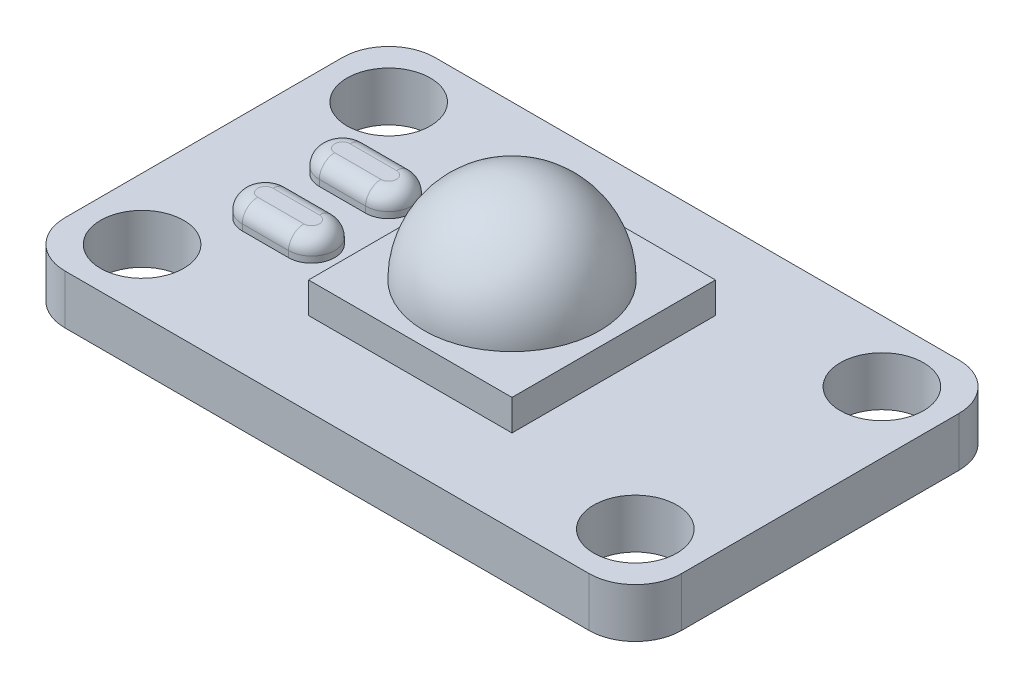
from build123d import *

# Parameters (mm, degrees)
EXTRUDE_375_DEPTH     = 1.6
SKETCH_7_R            = 1.35
CUT_EXTRUDE_535_DEPTH = 12.771151176
SKETCH_574_W          = 6.6
SKETCH_574_H          = 6.6
EXTRUDE_767_DEPTH     = 1
EXTRUDE_1228_DEPTH    = 0.7
EXTRUDE_1228_2_DEPTH  = 0.7
FILLET_1_R            = 0.5
FILLET_2_R            = 0.5


with BuildPart() as part:
    # Sketch 232 → Extrude 375 (new body)
    with BuildSketch(Plane(origin=(0, 0, 0), x_dir=(1, 0, 0), z_dir=(0, 1, 0))):
        with BuildLine():
            Line((-8.5, -6), (8.5, -6))
            ThreePointArc((8.5, -6), (9.560660172, -5.560660172), (10, -4.5))
            Line((10, -4.5), (10, 4.5))
            ThreePointArc((10, 4.5), (9.560660172, 5.560660172), (8.5, 6))
            Line((8.5, 6), (-8.5, 6))
            ThreePointArc((-8.5, 6), (-9.560660172, 5.560660172), (-10, 4.5))
            Line((-10, 4.5), (-10, -4.5))
            ThreePointArc((-10, -4.5), (-9.560660172, -5.560660172), (-8.5, -6))
        make_face()
    extrude(amount=EXTRUDE_375_DEPTH)

    # 草图7 → Cut-Extrude 535 (cut, through all)
    with BuildSketch(Plane(origin=(0, 0, 0), x_dir=(1, 0, 0), z_dir=(0, 1, 0))):
        with Locations(Location((-8, -4, 0), (0, 0, 270))):
            Circle(SKETCH_7_R)
        with Locations(Location((8, -4, 0), (0, 0, 270))):
            Circle(SKETCH_7_R)
        with Locations(Location((8, 4, 0), (0, 0, 270))):
            Circle(SKETCH_7_R)
        with Locations(Location((-8, 4, 0), (0, 0, 270))):
            Circle(SKETCH_7_R)
    extrude(amount=CUT_EXTRUDE_535_DEPTH, mode=Mode.SUBTRACT)


with BuildPart() as body_2:
    # Sketch 574 → Extrude 767 (new body)
    with BuildSketch(Plane(origin=(0, 1.6, 0), x_dir=(1, 0, 0), z_dir=(0, 1, 0))):
        Rectangle(SKETCH_574_W, SKETCH_574_H)
    extrude(amount=EXTRUDE_767_DEPTH)

    # Sketch 806 → Revolve 870 (revolve)
    with BuildSketch(Plane.XY):
        with BuildLine():
            Line((0, 2.6), (2.85, 2.6))
            ThreePointArc((2.85, 2.6), (2.015254326, 4.615254326), (0, 5.45))
            Line((0, 5.45), (0, 2.6))
        make_face()
    revolve(axis=Axis((0, 2.6, 0), (0, 1, 0)))


with BuildPart() as body_3:
    # Sketch 926 → Extrude 1228 (new body)
    with BuildSketch(Plane(origin=(0, 1.6, 0), x_dir=(1, 0, 0), z_dir=(0, 1, 0))):
        with BuildLine():
            Line((-6.75, 2), (-5.25, 2))
            ThreePointArc((-5.25, 2), (-4.5, 1.25), (-5.25, 0.5))
            Line((-5.25, 0.5), (-6.75, 0.5))
            ThreePointArc((-6.75, 0.5), (-7.5, 1.25), (-6.75, 2))
        make_face()
    extrude(amount=EXTRUDE_1228_DEPTH)

    # 焊点1
    fillet_1_edges = [body_3.edges().sort_by_distance(p)[0] for p in [
        (-4.5, 2.3, -1.25),
        (-6, 2.3, -2),
        (-7.5, 2.3, -1.25),
        (-6, 2.3, -0.5),
    ]]
    fillet(fillet_1_edges, radius=FILLET_1_R)


with BuildPart() as body_4:
    # Sketch 926 → Extrude 1228 2 (new body)
    with BuildSketch(Plane(origin=(0, 1.6, 0), x_dir=(1, 0, 0), z_dir=(0, 1, 0))):
        with BuildLine():
            Line((-6.75, -0.5), (-5.25, -0.5))
            ThreePointArc((-5.25, -0.5), (-4.5, -1.25), (-5.25, -2))
            Line((-5.25, -2), (-6.75, -2))
            ThreePointArc((-6.75, -2), (-7.5, -1.25), (-6.75, -0.5))
        make_face()
    extrude(amount=EXTRUDE_1228_2_DEPTH)

    # 焊点2
    fillet_2_edges = [body_4.edges().sort_by_distance(p)[0] for p in [
        (-7.5, 2.3, 1.25),
        (-6, 2.3, 2),
        (-4.5, 2.3, 1.25),
        (-6, 2.3, 0.5),
    ]]
    fillet(fillet_2_edges, radius=FILLET_2_R)


solid = Compound([part.part, body_2.part, body_3.part, body_4.part])
